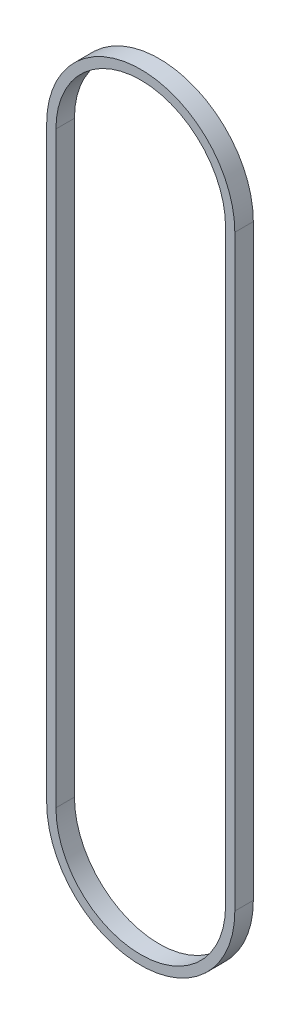
SolidWorks part; units mm, degrees
ref_plane "前视基准面" through (0, 0, 0) normal (0, 0, 1) x (1, 0, 0)
ref_plane "上视基准面" through (0, 0, 0) normal (0, 1, 0) x (1, 0, 0)
ref_plane "右视基准面" through (0, 0, 0) normal (1, 0, 0) x (0, 0, -1)
sketch "草图2" plane through (0, 0, 0) normal (0, 0, 1) x (1, 0, 0)
  line L0 (0, 0) -> (1, 0) construction
  line L1 (0, 0) -> (0, 1) construction
  line L2 (91.625, 0) -> (91.625, -635)
  line L3 (-91.625, -635) -> (-91.625, 0)
  arc A0 (-91.625, 0) -> (91.625, 0) centre (0, 0) cw
  arc A1 (91.625, -635) -> (-91.625, -635) centre (0, -635) cw
extrude "拉伸-薄壁1" add sketch "草图2" along normal mid plane 20 thin thin type one direction wall 10
